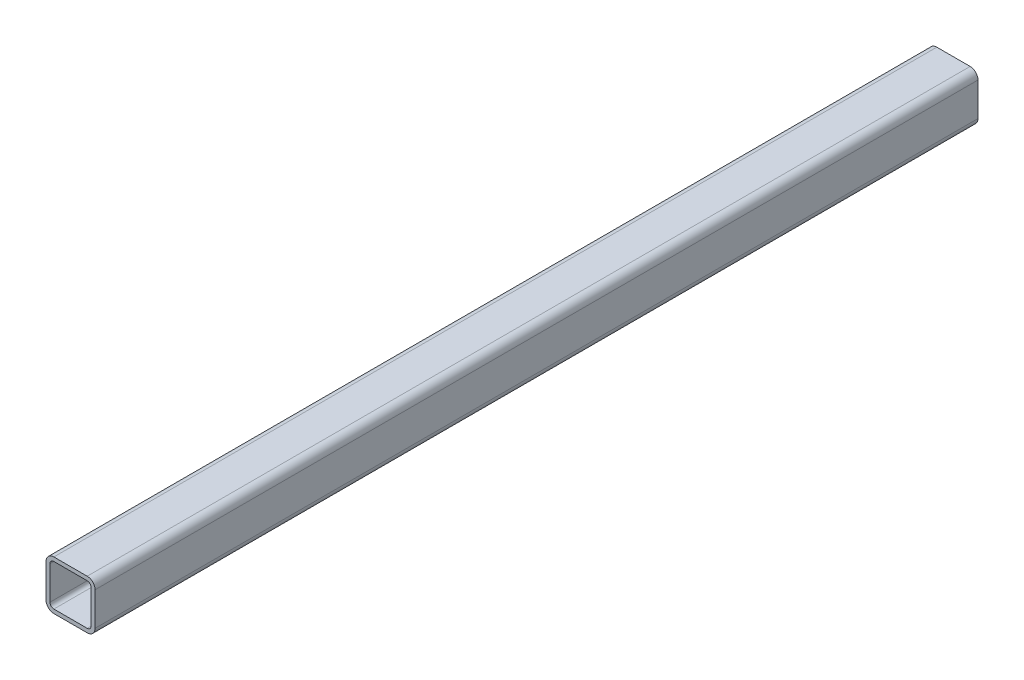
SolidWorks part; units mm, degrees
material "AISI 1045 钢，冷拔"
ref_plane "Front Plane" through (0, 0, 0) normal (0, 0, 1) x (1, 0, 0)
ref_plane "Top Plane" through (0, 0, 0) normal (0, 1, 0) x (1, 0, 0)
ref_plane "Right Plane" through (0, 0, 0) normal (1, 0, 0) x (0, 0, -1)
sketch "Sketch1" plane through (0, 0, 0) normal (0, 0, 1) x (1, 0, 0)
  line L0 (-21.0947, 0) -> (28.2454, 0) construction
  line L1 (0, 28.305) -> (0, -28.2454) construction
  line L2 (-17, 21) -> (17, 21)
  line L3 (-17, -25) -> (17, -25)
  line L4 (-25, -17) -> (-25, 17)
  line L5 (-17, 25) -> (17, 25)
  line L6 (25, -17) -> (25, 17)
  line L7 (-25, -25) -> (25, 25) construction
  line L8 (-25, 25) -> (25, -25) construction
  line L9 (21, -17) -> (21, 17)
  line L10 (-17, -21) -> (17, -21)
  line L11 (-21, -17) -> (-21, 17)
  arc A0 (17, -25) -> (25, -17) centre (17, -17) ccw
  arc A1 (-17, -25) -> (-25, -17) centre (-17, -17) cw
  arc A2 (17, 25) -> (25, 17) centre (17, 17) cw
  arc A3 (-25, 17) -> (-17, 25) centre (-17, 17) cw
  arc A4 (-21, 17) -> (-17, 21) centre (-17, 17) cw
  arc A5 (17, 21) -> (21, 17) centre (17, 17) cw
  arc A6 (17, -21) -> (21, -17) centre (17, -17) ccw
  arc A7 (-17, -21) -> (-21, -17) centre (-17, -17) cw
  point P5 (0, 0)
  dimension "D3" = 8
  dimension "D1" = 50
  dimension "D2" = 50
  dimension "D4" = 4
extrude "Boss-Extrude1" add sketch "Sketch1" along normal mid plane 900
